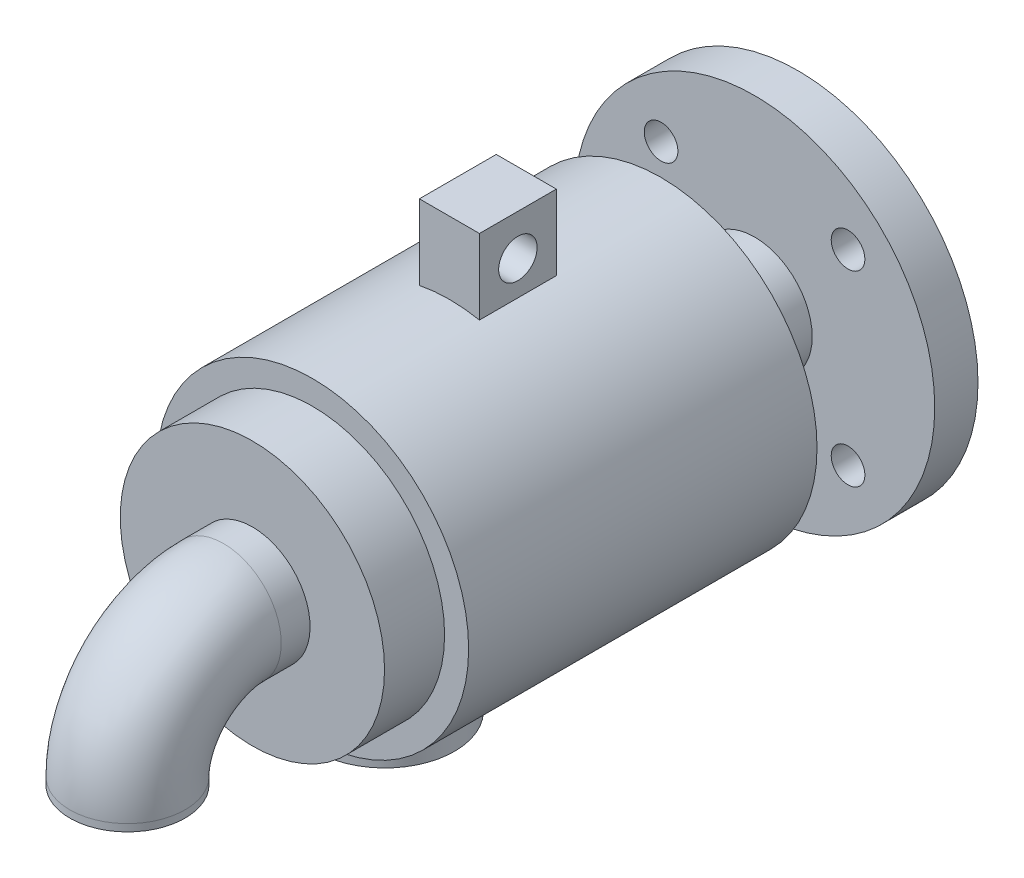
from build123d import *

# Parameters (mm, degrees)
SKETCH1_R             = 75
BOSS_EXTRUDE1_DEPTH   = 18
SKETCH2_R             = 24
CUT_EXTRUDE1_DEPTH    = 12
SKETCH5_R             = 24
SKETCH6_R             = 65
BOSS_EXTRUDE2_DEPTH   = 170
F_14_0_14_HOLE1_D     = 14
F_14_0_14_HOLE1_DEPTH = 18
CIRPATTERN1_COUNT     = 4
SKETCH10_R            = 29
BOSS_EXTRUDE3_DEPTH   = 70
SKETCH11_R            = 19
CUT_EXTRUDE2_DEPTH    = 187
SKETCH13_R            = 12.5
CUT_EXTRUDE3_START    = -25
SKETCH14_R            = 65
SKETCH14_R_2          = 55
CUT_EXTRUDE3_DEPTH    = 25
SKETCH15_R            = 24
CUT_EXTRUDE4_DEPTH    = 60
SKETCH16_W            = 32
SKETCH16_H            = 71.063102747
BOSS_EXTRUDE4_DEPTH   = 12.5
SKETCH17_R            = 8
CUT_EXTRUDE5_DEPTH    = 25


with BuildPart() as part:
    # Sketch1 → Boss-Extrude1 (new body)
    with BuildSketch(Plane.XY):
        Circle(SKETCH1_R)
    extrude(amount=BOSS_EXTRUDE1_DEPTH)

    # Sketch2 → Cut-Extrude1 (cut)
    with BuildSketch(Plane.XY.offset(18)):
        Circle(SKETCH2_R)
    extrude(amount=-CUT_EXTRUDE1_DEPTH, mode=Mode.SUBTRACT)

    # Sweep1: sweep along a path in Sketch3
    with BuildLine(Plane(origin=(0, 0, 0), x_dir=(0, 0, -1), z_dir=(1, 0, 0))) as sweep1_path:
        Line((12, 0), (-239, 0))
        ThreePointArc((-239, 0), (-267.284271247, -11.715728753), (-279, -40))
        Line((-279, -40), (-279, -43))
    # Sketch5 → Sweep1 (sweep)
    with BuildSketch(Plane(origin=(0, 0, -12), x_dir=(-1, 0, 0), z_dir=(0, 0, -1))):
        Circle(SKETCH5_R)
    sweep(path=sweep1_path.line)

    # Sketch6 → Boss-Extrude2 (add)
    with BuildSketch(Plane(origin=(0, 0, 57), x_dir=(-1, 0, 0), z_dir=(0, 0, -1))):
        Circle(SKETCH6_R)
    extrude(amount=-BOSS_EXTRUDE2_DEPTH)

    # Ø14.0 (14) Hole1
    with Locations(Plane(origin=(0, 0, 0), x_dir=(-1, 0, 0), z_dir=(0, 0, -1))):
        with Locations((-38.905866791, 38.905866791)):
            f_14_0_14_hole1 = Hole(F_14_0_14_HOLE1_D / 2, depth=F_14_0_14_HOLE1_DEPTH)

    # CirPattern1: Ø14.0 (14) Hole1 ×4 about axis
    cirpattern1_axis = Axis((0, 0, 0), (0, 0, 1))
    for i in range(1, CIRPATTERN1_COUNT):
        add(f_14_0_14_hole1.rotate(cirpattern1_axis, i * 360 / CIRPATTERN1_COUNT), mode=Mode.SUBTRACT)

    # Sketch10 → Boss-Extrude3 (add)
    with BuildSketch(Plane(origin=(0, 0, 0), x_dir=(1, 0, 0), z_dir=(0, 1, 0))):
        with Locations(Location((0, -171.843858555, 0), (0, 0, 270))):
            Circle(SKETCH10_R)
    extrude(amount=-BOSS_EXTRUDE3_DEPTH)

    # Sketch11 → Cut-Extrude2 (cut)
    with BuildSketch(Plane(origin=(0, 0, -12), x_dir=(-1, 0, 0), z_dir=(0, 0, -1))):
        Circle(SKETCH11_R)
    extrude(amount=-CUT_EXTRUDE2_DEPTH, mode=Mode.SUBTRACT)

    # Cut-Sweep1: sweep along a path in Sketch12
    with BuildLine(Plane(origin=(0, 0, 0), x_dir=(0, 0, -1), z_dir=(1, 0, 0))) as cut_sweep1_path:
        Line((-279, -43), (-279, -30))
        ThreePointArc((-279, -30), (-270.213203436, -8.786796564), (-249, 0))
        Line((-249, 0), (-239, 0))
    # Sketch13 → Cut-Sweep1 (sweep, cut)
    with BuildSketch(Plane.XZ.offset(43)):
        with Locations((0, 279)):
            Circle(SKETCH13_R)
    sweep(path=cut_sweep1_path.line, mode=Mode.SUBTRACT)

    # Sketch14 → Cut-Extrude3 (cut)
    with BuildSketch(Plane.XY.offset(227).offset(CUT_EXTRUDE3_START)):
        with Locations(Location((0, 0, 0), (0, 0, 180))):
            Circle(SKETCH14_R)
        Circle(SKETCH14_R_2, mode=Mode.SUBTRACT)
    extrude(amount=CUT_EXTRUDE3_DEPTH, mode=Mode.SUBTRACT)

    # Sketch15 → Cut-Extrude4 (cut)
    with BuildSketch(Plane(origin=(0, -70, 0), x_dir=(-1, 0, 0), z_dir=(0, -1, 0))):
        with Locations(Location((0, -171.843858555, 0), (0, 0, 90))):
            Circle(SKETCH15_R)
    extrude(amount=-CUT_EXTRUDE4_DEPTH, mode=Mode.SUBTRACT)

    # Sketch16 → Boss-Extrude4 (add, symmetric)
    with BuildSketch(Plane(origin=(0, 0, 0), x_dir=(0, 0, -1), z_dir=(1, 0, 0))):
        with Locations((-129, 59.468448626)):
            Rectangle(SKETCH16_W, SKETCH16_H)
    extrude(amount=BOSS_EXTRUDE4_DEPTH, both=True)

    # Sketch17 → Cut-Extrude5 (cut)
    with BuildSketch(Plane(origin=(12.5, 0, 0), x_dir=(0, 0, -1), z_dir=(1, 0, 0))):
        with Locations((-129, 78)):
            Circle(SKETCH17_R)
    extrude(amount=-CUT_EXTRUDE5_DEPTH, mode=Mode.SUBTRACT)


solid = part.part
